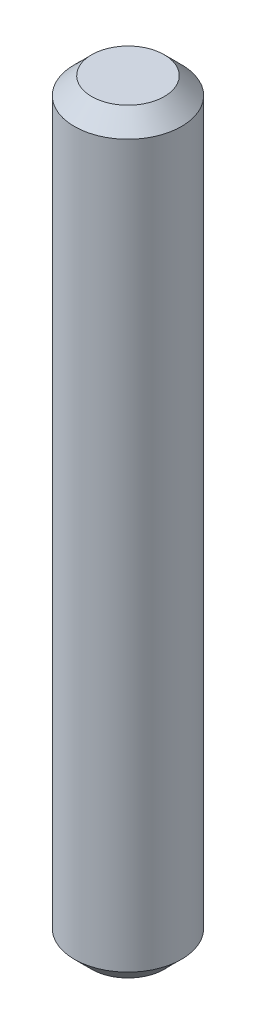
SolidWorks part; units mm, degrees
material "AISI 4130 Steel, normalized at 870C"
ref_plane "Front" through (0, 0, 0) normal (0, 0, 1) x (1, 0, 0)
ref_plane "Top" through (0, 0, 0) normal (0, 1, 0) x (1, 0, 0)
ref_plane "Right" through (0, 0, 0) normal (1, 0, 0) x (0, 0, -1)
sketch "Sketch1" plane through (0, 0, 0) normal (0, 1, 0) x (1, 0, 0)
  circle A0 centre (0, 0) radius 0.7874
  dimension "D1" = 1.5748
extrude "Boss-Extrude1" add sketch "Sketch1" along normal blind 11.1125
chamfer "Chamfer1" distance 0.254 angle 45 2 edges at (0, 11.1125, 0.7874) (0, 0, 0.7874)
